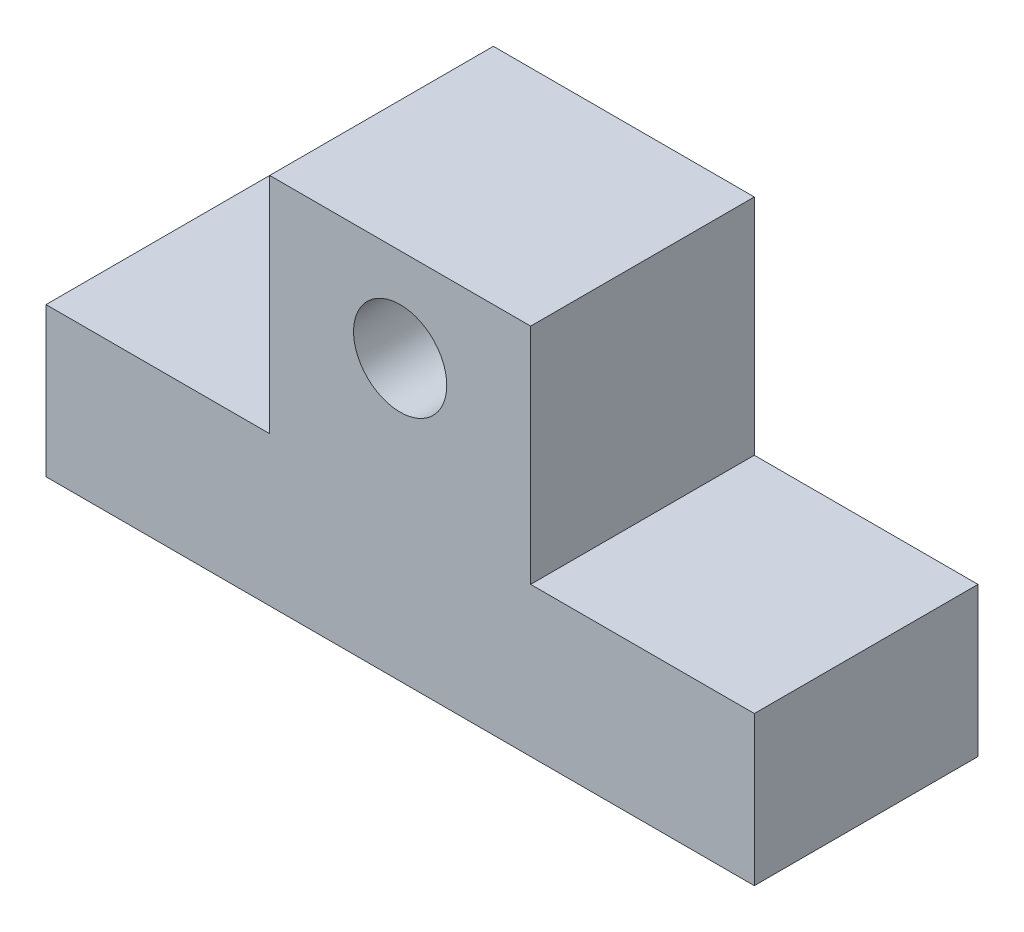
SolidWorks part; units mm, degrees
ref_plane "前视基准面" through (0, 0, 0) normal (0, 0, 1) x (1, 0, 0)
ref_plane "上视基准面" through (0, 0, 0) normal (0, 1, 0) x (1, 0, 0)
ref_plane "右视基准面" through (0, 0, 0) normal (1, 0, 0) x (0, 0, -1)
sketch "草图1" plane through (0, 0, 0) normal (0, 0, 1) x (1, 0, 0)
  line L0 (0, 0) -> (-7, 0)
  line L1 (-7, 0) -> (-7, -12)
  line L2 (-7, -12) -> (-19, -12)
  line L3 (-19, -12) -> (-19, -20)
  line L4 (-19, -20) -> (19, -20)
  line L5 (19, -20) -> (19, -12)
  line L6 (19, -12) -> (7, -12)
  line L7 (7, -12) -> (7, 0)
  line L8 (7, 0) -> (0, 0)
  dimension "D1" = 14
  dimension "D2" = 8
  dimension "D3" = 12
  dimension "D4" = 12
extrude "凸台-拉伸1" add sketch "草图1" along normal mid plane 12
hole_wizard "M6 螺纹孔1" positions "3D草图1" profile "草图2" tap size "M6" standard "GB" end condition up to next
sketch3d "3D草图1"
  line L0 (-19, -20, 6) -> (19, -20, 6) construction
  line L1 (0, -20, 6) -> (0, -5, 6) construction
  point P0 (0, -5, 6)
  dimension "D1" = 15
sketch "草图2" plane through (0, -5, 6) normal (1, 0, 0) x (0, -1, 0)
  line L0 (0, 0) -> (0, 12)
  line L1 (0, 12) -> (2.5, 12)
  line L2 (2.5, 12) -> (2.5, 0)
  line L5 (2.5, 0) -> (0, 0)
  line L11 (0, -6.35) -> (0, 107.95) construction
  dimension "通孔螺纹孔钻头直径" = 5
  dimension "通孔螺纹孔钻头深度" = 12
cosmetic thread "孔螺蚊线1"
